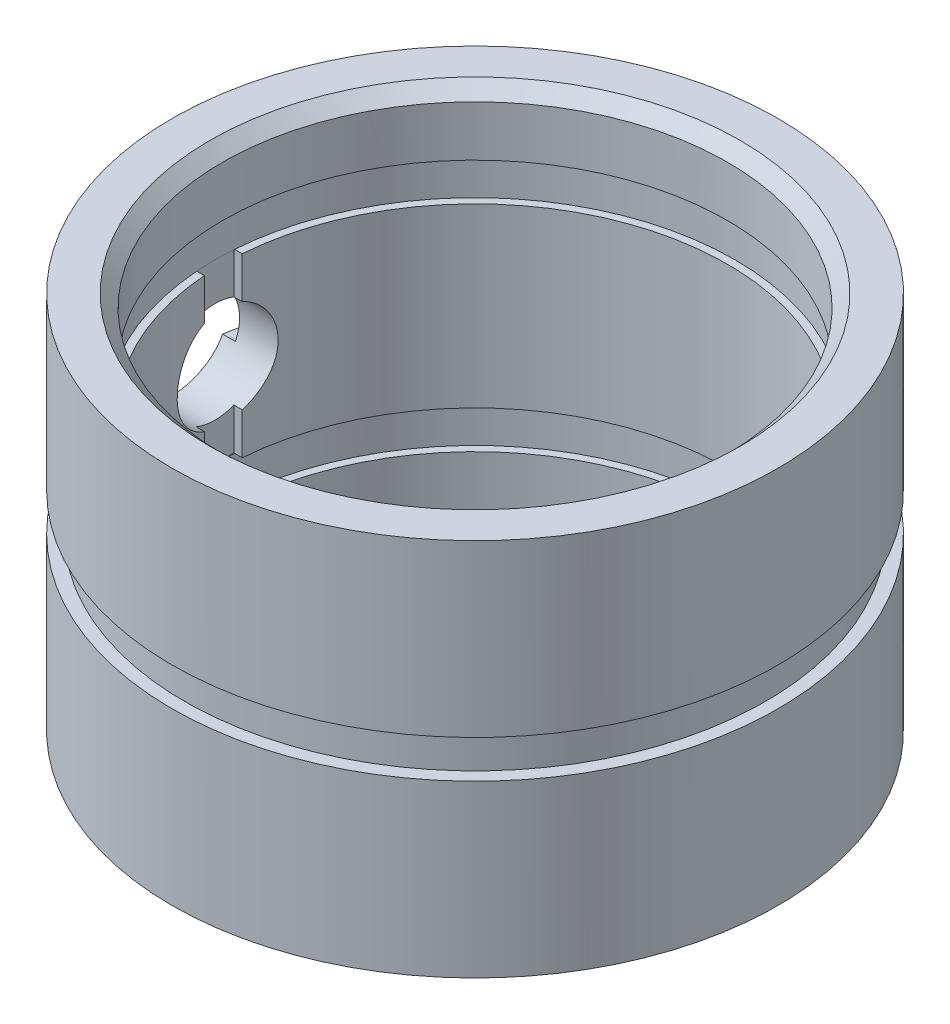
SolidWorks part; units mm, degrees
material "铜"
ref_plane "前视基准面" through (0, 0, 0) normal (0, 0, 1) x (1, 0, 0)
ref_plane "上视基准面" through (0, 0, 0) normal (0, 1, 0) x (1, 0, 0)
ref_plane "右视基准面" through (0, 0, 0) normal (1, 0, 0) x (0, 0, -1)
sketch "草图1" plane through (0, 0, 0) normal (0, 1, 0) x (1, 0, 0)
  circle A0 centre (0, 0) radius 20
  circle A1 centre (0, 0) radius 24
  dimension "D1" = 40
  dimension "D2" = 48
extrude "凸台-拉伸1" add sketch "草图1" along normal mid plane 30
sketch "草图2" plane through (0, 0, 0) normal (0, 0, 1) x (1, 0, 0)
  line L0 (-37.4763, 0) -> (34.2216, 0) construction
  line L1 (0, 33.8873) -> (0, -35.0792) construction
  line L2 (20, 15) -> (-20, 15) construction
  line L3 (0, 10) -> (20.6, 10)
  line L4 (0, 10) -> (0, 7)
  line L5 (0, 7) -> (20.6, 7)
  line L6 (20.6, 10) -> (20.6, 7)
  line L7 (20.6, -10) -> (20.6, -7)
  line L8 (0, -7) -> (20.6, -7)
  line L9 (0, -10) -> (0, -7)
  line L10 (0, -10) -> (20.6, -10)
  line L12 (23, 1.5) -> (27.5, 1.5)
  line L13 (23, 1.5) -> (23, -1.5)
  line L14 (23, -1.5) -> (27.5, -1.5)
  line L15 (27.5, 1.5) -> (27.5, -1.5)
  dimension "D1" = 5
  dimension "D2" = 3
  dimension "D3" = 41.2
  dimension "D4" = 46
  dimension "D5" = 3
  dimension "D6" = 55
revolve "切除-旋转1" cut sketch "草图2" angle 360 about L1
sketch "草图5" plane through (0, 0, 0) normal (0, 1, 0) x (1, 0, 0)
  line L0 (-27.4217, 0) -> (26.9262, 0) construction
  line L1 (0, 16.5747) -> (0, -7.9882) construction
  line L2 (17.5, 1.5) -> (17.5, -1.5)
  line L3 (-20.6, 1.5) -> (-17.5, 1.5)
  line L4 (-20.6, 1.5) -> (-20.6, -1.5)
  line L5 (-20.6, -1.5) -> (-17.5, -1.5)
  line L6 (-17.5, 1.5) -> (-17.5, -1.5)
  line L7 (20.6, -1.5) -> (17.5, -1.5)
  line L8 (20.6, 1.5) -> (20.6, -1.5)
  line L9 (20.6, 1.5) -> (17.5, 1.5)
  dimension "D1" = 41.2
  dimension "D2" = 35
  dimension "D3" = 3
extrude "切除-拉伸1" cut sketch "草图5" against normal mid plane 14
sketch "草图6" plane through (0, 0, 0) normal (1, 0, 0) x (0, 0, -1)
  circle A0 centre (0, 0) radius 4
  dimension "D1" = 8
extrude "切除-拉伸2" cut sketch "草图6" against normal through all
chamfer "倒角1" distance 1 angle 45 2 edges at (0, -15, 20) (0, 15, 20)
